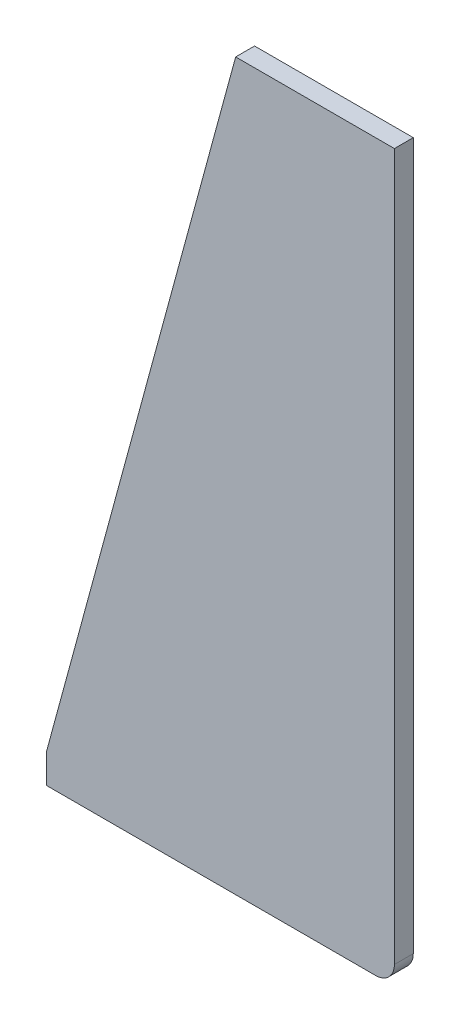
SolidWorks part; units mm, degrees
material "1023 Carbon steel plate (SS)"
ref_plane "Front Plane" through (0, 0, 0) normal (0, 0, 1) x (1, 0, 0)
ref_plane "Top Plane" through (0, 0, 0) normal (0, 1, 0) x (1, 0, 0)
ref_plane "Right Plane" through (0, 0, 0) normal (1, 0, 0) x (0, 0, -1)
sketch "Sketch1" plane through (0, 0, 0) normal (0, 0, 1) x (1, 0, 0)
  line L0 (0, 0) -> (-50, -184)
  line L1 (-50, -184) -> (-50, -192)
  line L2 (-50, -192) -> (37, -192)
  line L3 (42, -187) -> (42, 0)
  line L4 (42, 0) -> (0, 0)
  arc A0 (37, -192) -> (42, -187) centre (37, -187) ccw
  dimension "D3" = 5
  dimension "D1" = 42
  dimension "D2" = 192
  dimension "D4" = 92
  dimension "D5" = 8
extrude "Boss-Extrude1" add sketch "Sketch1" along normal blind 5 contours L4 L0 L1 L2 A0 L3
